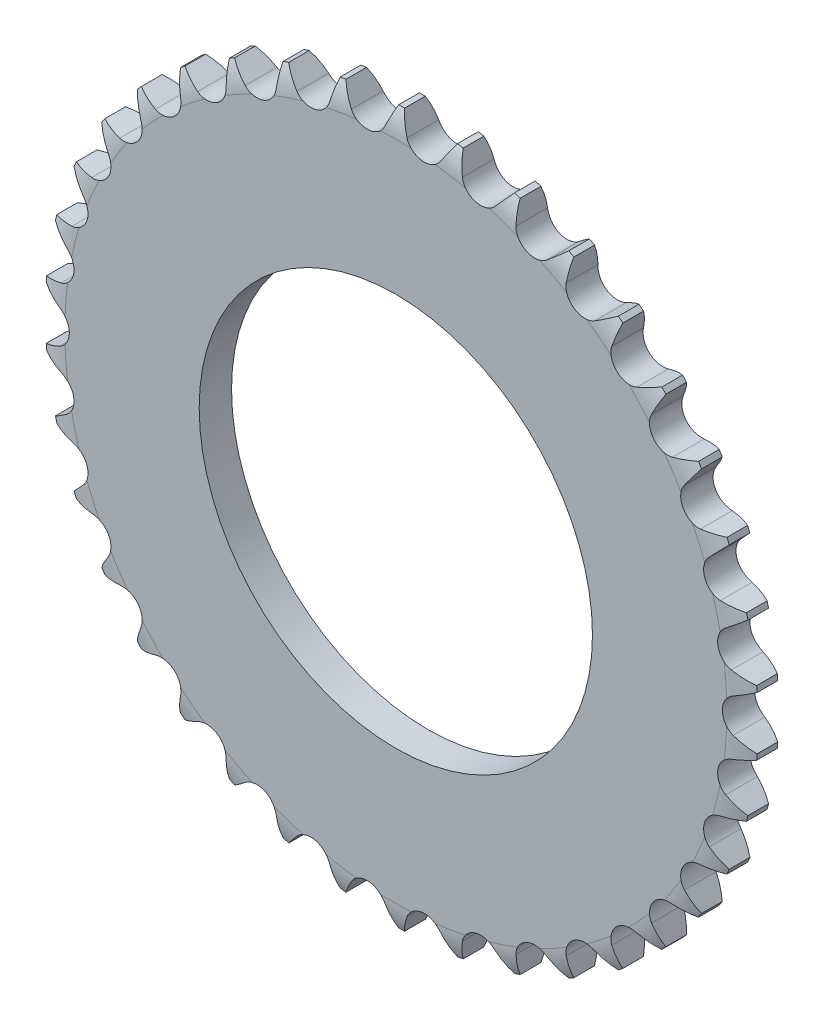
from build123d import *

# Parameters (mm, degrees)
CUT_EXTRUDE_1_DEPTH      = 118.481828382
PATTERN_CIRCULAR_1_COUNT = 38


with BuildPart() as part:
    # 草图4 → 旋转1 (revolve)
    with BuildSketch(Plane(origin=(0, 0, 0), x_dir=(0, 0, -1), z_dir=(1, 0, 0))):
        with BuildLine():
            Line((-35, 43.75), (-27.8, 43.75))
            Line((-27.8, 43.75), (-27.8, 73.633431373))
            ThreePointArc((-27.8, 73.633431373), (-28.129167352, 76.540319744), (-29.1, 79.3))
            Line((-29.1, 79.3), (-33.7, 79.3))
            ThreePointArc((-33.7, 79.3), (-34.670832648, 76.540319744), (-35, 73.633431373))
            Line((-35, 73.633431373), (-35, 43.75))
        make_face()
    revolve(axis=Axis((0, 0, 0), (0, 0, 1)))

    # 草图5 → 切除-拉伸1 (cut, through all)
    with BuildSketch(Plane.XY):
        with BuildLine():
            Line((0.65, 79.297336021), (2.416505089, 75.014834577))
            ThreePointArc((2.416505089, 75.014834577), (5.998644343, 72.396908021), (9.962806149, 74.389565109))
            Line((9.962806149, 74.389565109), (12.410058883, 78.322924093))
            ThreePointArc((12.410058883, 78.322924093), (6.548179454, 79.029180344), (0.65, 79.297336021))
        make_face()
    cut_extrude_1 = extrude(amount=CUT_EXTRUDE_1_DEPTH, mode=Mode.SUBTRACT)

    # 阵列(圆周)1: 切除-拉伸1 ×38 about axis
    pattern_circular_1_axis = Axis((0, 0, 0), (0, 0, 1))
    for i in range(1, PATTERN_CIRCULAR_1_COUNT):
        add(cut_extrude_1.rotate(pattern_circular_1_axis, i * 360 / PATTERN_CIRCULAR_1_COUNT), mode=Mode.SUBTRACT)


solid = part.part
